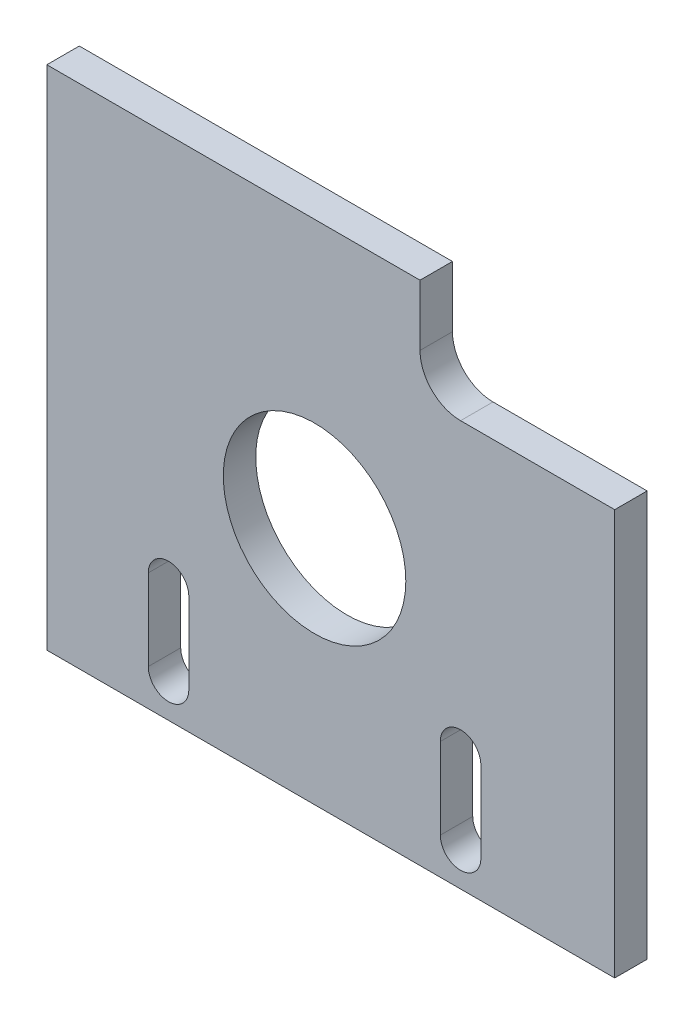
from build123d import *

# Parameters (mm, degrees)
SKETCH1_W           = 140
SKETCH1_H           = 125
BOSS_EXTRUDE1_DEPTH = 8
SKETCH2_R           = 22.5
CUT_EXTRUDE1_DEPTH  = 8
CUT_EXTRUDE2_DEPTH  = 8
LPATTERN1_COUNT     = 2
LPATTERN1_PITCH     = 72
SKETCH4_W           = 48
SKETCH4_H           = 25
CUT_EXTRUDE3_DEPTH  = 8
FILLET1_R           = 10


with BuildPart() as part:
    # Sketch1 → Boss-Extrude1 (new body)
    with BuildSketch(Plane.XY):
        with Locations((70, -62.5)):
            Rectangle(SKETCH1_W, SKETCH1_H)
    extrude(amount=BOSS_EXTRUDE1_DEPTH)

    # Sketch2 → Cut-Extrude1 (cut)
    with BuildSketch(Plane.XY.offset(8)):
        with Locations((66, -66)):
            Circle(SKETCH2_R)
    extrude(amount=-CUT_EXTRUDE1_DEPTH, mode=Mode.SUBTRACT)

    # Sketch3 → Cut-Extrude2 (cut)
    with BuildSketch(Plane.XY.offset(8)):
        with BuildLine():
            Line((35, -96), (35, -116))
            ThreePointArc((35, -116), (30, -121), (25, -116))
            Line((25, -116), (25, -96))
            ThreePointArc((25, -96), (30, -91), (35, -96))
        make_face()
    cut_extrude2 = extrude(amount=-CUT_EXTRUDE2_DEPTH, mode=Mode.SUBTRACT)

    # LPattern1: Cut-Extrude2 ×2
    with Locations(*[(i * LPATTERN1_PITCH, 0, 0) for i in range(1, LPATTERN1_COUNT)]):
        add(cut_extrude2, mode=Mode.SUBTRACT)

    # Sketch4 → Cut-Extrude3 (cut)
    with BuildSketch(Plane.XY.offset(8)):
        with Locations((116, -12.5)):
            Rectangle(SKETCH4_W, SKETCH4_H)
    extrude(amount=-CUT_EXTRUDE3_DEPTH, mode=Mode.SUBTRACT)

    # Fillet1
    fillet1_edges = [part.edges().sort_by_distance(p)[0] for p in [
        (92, -25, 4),
    ]]
    fillet(fillet1_edges, radius=FILLET1_R)


solid = part.part
